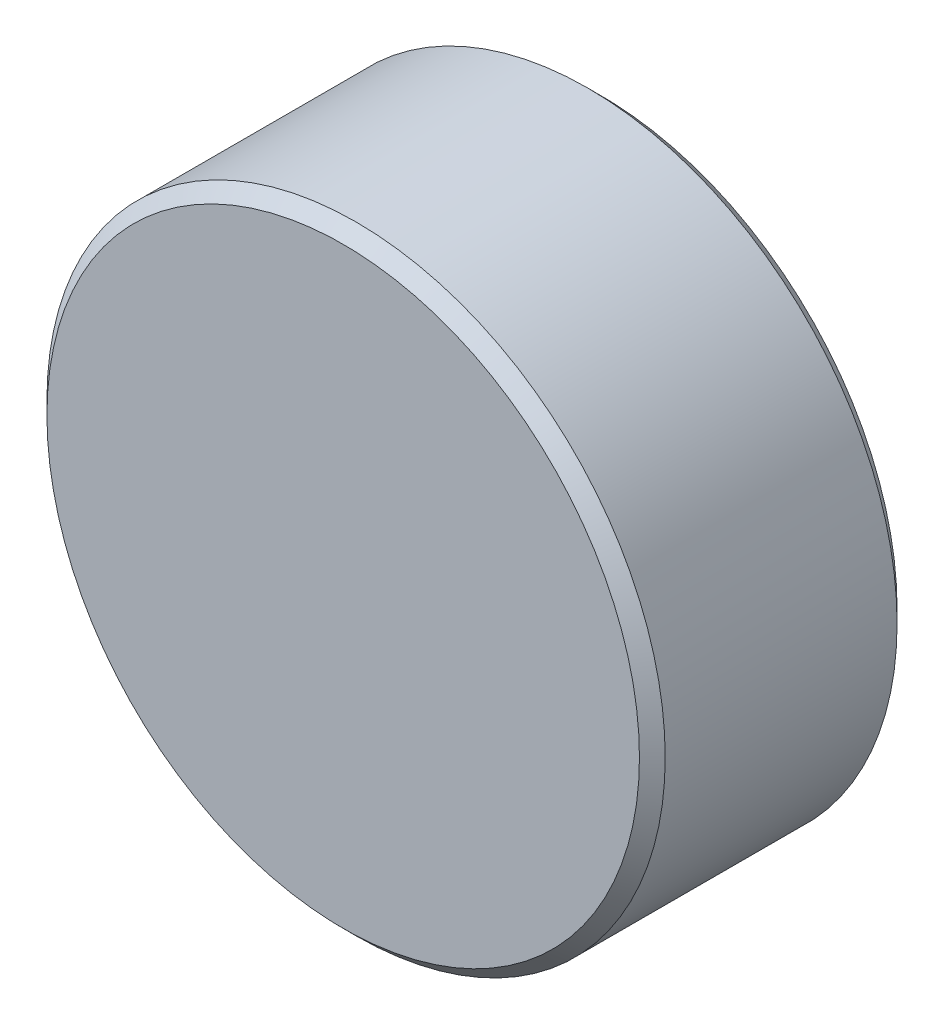
from build123d import *

# Parameters (mm, degrees)
SKETCH_1_R          = 12
EXTRUDE_1_DEPTH     = 10
CHAMFER_1_SIZE      = 0.5
CUT_EXTRUDE_1_DEPTH = 8


with BuildPart() as part:
    # 草图1 → 凸台-拉伸1 (new body)
    with BuildSketch(Plane.XY):
        Circle(SKETCH_1_R)
    extrude(amount=EXTRUDE_1_DEPTH)

    # 倒角1
    chamfer_1_edges = [part.edges().sort_by_distance(p)[0] for p in [
        (-12, 0, 0),
        (-12, 0, 10),
    ]]
    chamfer(chamfer_1_edges, length=CHAMFER_1_SIZE)

    # 草图2 → 切除-拉伸1 (cut)
    with BuildSketch(Plane(origin=(0, 0, 0), x_dir=(-1, 0, 0), z_dir=(0, 0, -1))):
        Polygon((0, -3.464101615), (3, -1.732050808), (3, 1.732050808), (0, 3.464101615), (-3, 1.732050808), (-3, -1.732050808), align=None)
    extrude(amount=-CUT_EXTRUDE_1_DEPTH, mode=Mode.SUBTRACT)


solid = part.part
